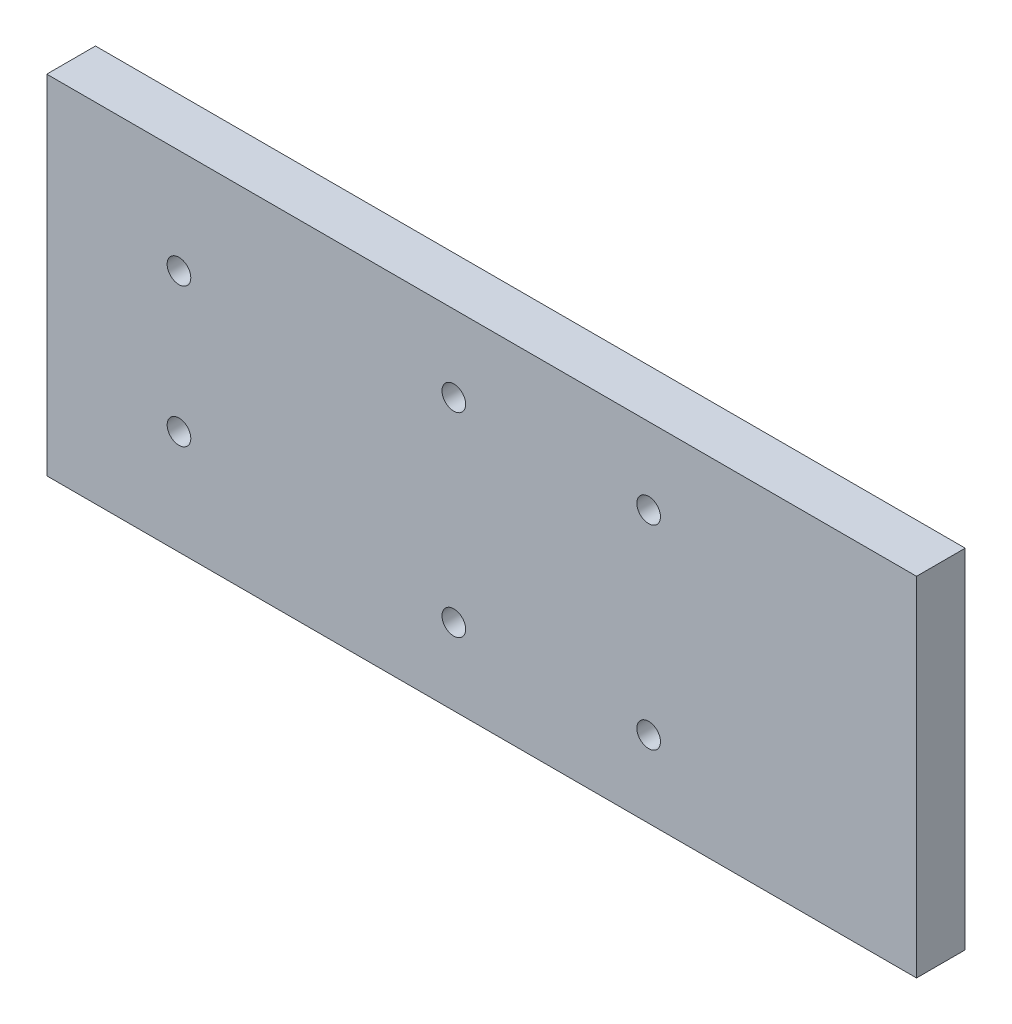
from build123d import *

# Parameters (mm, degrees)
SKETCH1_W             = 250
SKETCH1_H             = 100
SKETCH1_R             = 2.5
BOSS_EXTRUDE1_DEPTH   = 14
M8_TAPPED_HOLE1_D     = 6.8
M8_TAPPED_HOLE1_DEPTH = 19.75
M8_TAPPED_HOLE1_TIP   = 2.042926105
M8_TAPPED_HOLE2_D     = 6.8


with BuildPart() as part:
    # Sketch1 → Boss-Extrude1 (new body)
    with BuildSketch(Plane.XY):
        with Locations((125, 50)):
            Rectangle(SKETCH1_W, SKETCH1_H)
        with Locations((117, 78)):
            Circle(SKETCH1_R, mode=Mode.SUBTRACT)
        with Locations((173, 78)):
            Circle(SKETCH1_R, mode=Mode.SUBTRACT)
        with Locations((117, 22)):
            Circle(SKETCH1_R, mode=Mode.SUBTRACT)
        with Locations((173, 22)):
            Circle(SKETCH1_R, mode=Mode.SUBTRACT)
    extrude(amount=BOSS_EXTRUDE1_DEPTH)

    # M8 Tapped Hole1
    with Locations(Plane.XY.offset(14)):
        with Locations((117, 78), (173, 78), (117, 22), (173, 22)):
            Hole(M8_TAPPED_HOLE1_D / 2, depth=M8_TAPPED_HOLE1_DEPTH)
            with Locations((0, 0, -(M8_TAPPED_HOLE1_DEPTH + M8_TAPPED_HOLE1_TIP / 2))):  # 118° drill point
                Cone(0, M8_TAPPED_HOLE1_D / 2, M8_TAPPED_HOLE1_TIP, mode=Mode.SUBTRACT)

    # M8 Tapped Hole2 (through all)
    with Locations(Plane.XY.offset(14)):
        with Locations((38, 70), (38, 30)):
            Hole(M8_TAPPED_HOLE2_D / 2)


solid = part.part
